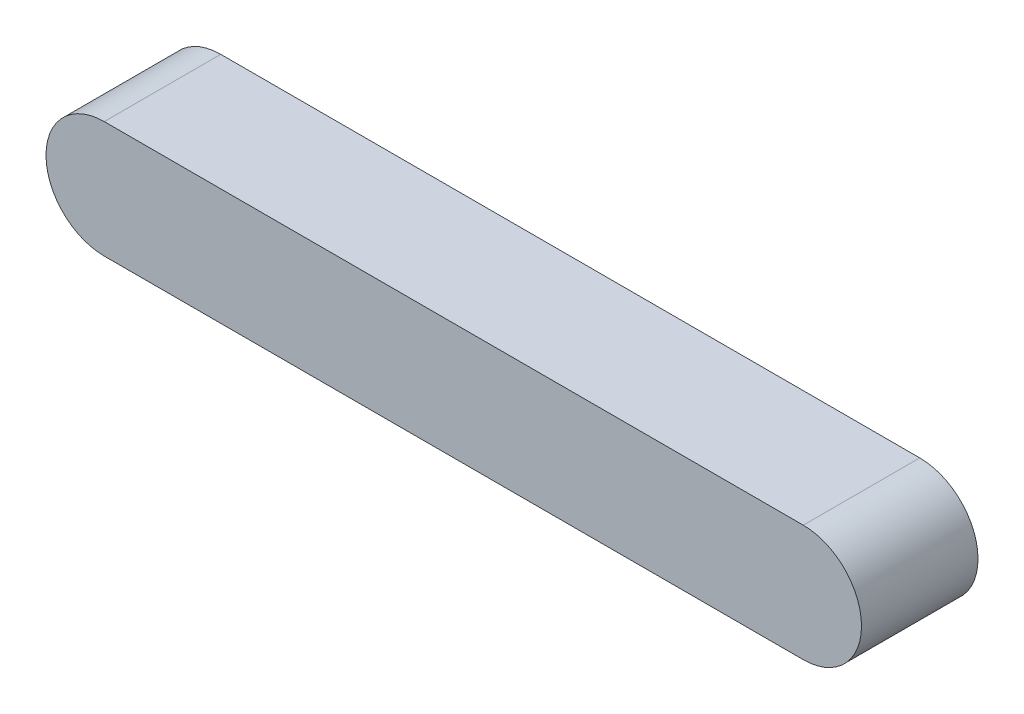
from build123d import *

# Parameters (mm, degrees)
BOSS_EXTRUDE1_DEPTH = 5


with BuildPart() as part:
    # Sketch1 → Boss-Extrude1 (new body)
    with BuildSketch(Plane.XY):
        with BuildLine():
            Line((-15, 2.5), (15, 2.5))
            ThreePointArc((15, 2.5), (17.5, 0), (15, -2.5))
            Line((15, -2.5), (-15, -2.5))
            ThreePointArc((-15, -2.5), (-17.5, 0), (-15, 2.5))
        make_face()
    extrude(amount=BOSS_EXTRUDE1_DEPTH)


solid = part.part
